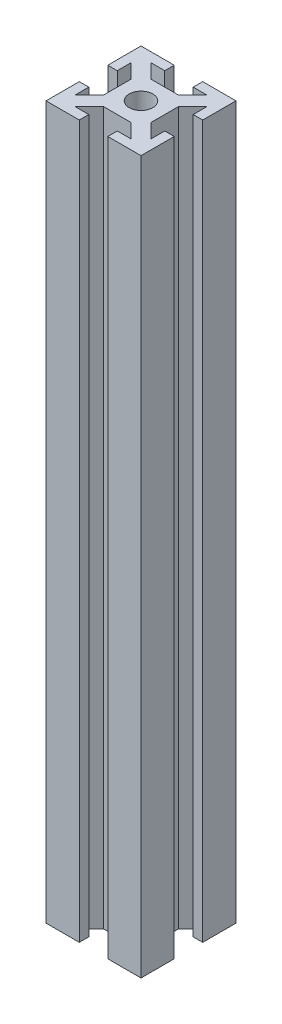
from build123d import *

# Parameters (mm, degrees)
SKETCH1_R           = 5
BOSS_EXTRUDE1_DEPTH = 300


with BuildPart() as part:
    # Sketch1 → Boss-Extrude1 (new body)
    with BuildSketch(Plane(origin=(0, 0, 0), x_dir=(1, 0, 0), z_dir=(0, 1, 0))):
        Polygon((-6, 20), (-6, 16), (-11.757359313, 16), (-5.757359313, 10), (5.757359313, 10), (11.757359313, 16), (6, 16), (6, 20), (20, 20), (20, 6), (16, 6), (16, 11.757359313), (10, 5.757359313), (10, -5.757359313), (16, -11.757359313), (16, -6), (20, -6), (20, -20), (6, -20), (6, -16), (11.757359313, -16), (5.757359313, -10), (-5.757359313, -10), (-11.757359313, -16), (-6, -16), (-6, -20), (-20, -20), (-20, -6), (-16, -6), (-16, -11.757359313), (-10, -5.757359313), (-10, 5.757359313), (-16, 11.757359313), (-16, 6), (-20, 6), (-20, 20), align=None)
        with Locations(Location((0, 0, 0), (0, 0, 270))):
            Circle(SKETCH1_R, mode=Mode.SUBTRACT)
    extrude(amount=BOSS_EXTRUDE1_DEPTH)


solid = part.part
